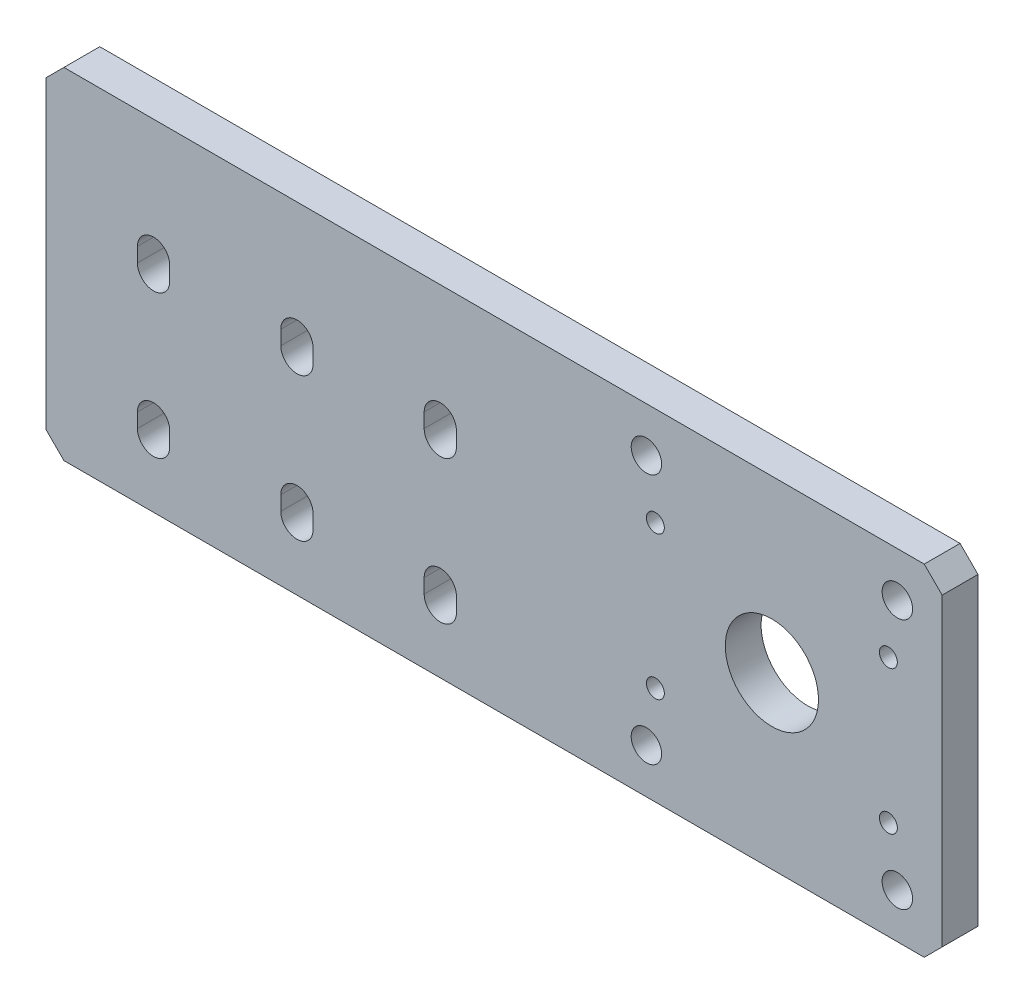
SolidWorks part; units mm, degrees
material "AISI 1045 钢，冷拔"
ref_plane "前视基准面" through (0, 0, 0) normal (0, 0, 1) x (1, 0, 0)
ref_plane "上视基准面" through (0, 0, 0) normal (0, 1, 0) x (1, 0, 0)
ref_plane "右视基准面" through (0, 0, 0) normal (1, 0, 0) x (0, 0, -1)
sketch "草图1" plane through (0, 0, 0) normal (0, 0, 1) x (1, 0, 0)
  line L1 (-125, 47.5) -> (125, 47.5)
  line L2 (-125, 47.5) -> (-125, -47.5)
  line L3 (-125, -47.5) -> (125, -47.5)
  line L4 (125, 47.5) -> (125, -47.5)
  line L5 (-125, 47.5) -> (125, -47.5) construction
  line L6 (-125, -47.5) -> (125, 47.5) construction
  point P0 (0, 0)
  dimension "D1" = 95
  dimension "D2" = 250
extrude "凸台-拉伸1" add sketch "草图1" along normal blind 10
sketch "草图3" plane through (0, 0, 10) normal (0, 0, 1) x (1, 0, 0)
  line L0 (-55, 17.5058) -> (-55, -69.5405) construction
  line L1 (125, -47.5) -> (125, 47.5) construction
  line L2 (-22.9727, -29.5) -> (-57.0867, -29.5) construction
  line L3 (-125, -47.5) -> (125, -47.5) construction
  line L4 (-55, -29.5) -> (-55, -25.5) construction
  line L5 (-59.5, -29.5) -> (-59.5, -25.5)
  line L6 (-50.5, -29.5) -> (-50.5, -25.5)
  arc A0 (-59.5, -29.5) -> (-50.5, -29.5) centre (-55, -29.5) ccw
  arc A1 (-50.5, -25.5) -> (-59.5, -25.5) centre (-55, -25.5) ccw
  point P10 (-55, -27.5)
  dimension "D4" = 4.5
  dimension "D1" = 180
  dimension "D2" = 18
  dimension "D3" = 4
extrude "切除-拉伸2" cut sketch "草图3" against normal through all
pattern_linear "阵列(线性)1" count 2 spacing 40 along (1, 0, 0) count 2 spacing 40 along (0, 1, 0) of "切除-拉伸2"
pattern_linear "阵列(线性)2" count 2 spacing 40 along (-1, 0, 0) count 2 spacing 40 along (0, 1, 0) of "切除-拉伸2"
chamfer "倒角1" distance 5 angle 45 4 edges at (125, -47.5, 5) (125, 47.5, 5) (-125, -47.5, 5) (-125, 47.5, 5)
sketch "草图10" plane through (0, 0, 10) normal (0, 0, 1) x (1, 0, 0)
  line L0 (5.5, 0) -> (-5.5, 0) construction
  line L1 (42.5, 35) -> (112.5, 35) construction
  line L2 (42.5, 35) -> (42.5, -35) construction
  line L3 (42.5, -35) -> (112.5, -35) construction
  line L4 (112.5, 35) -> (112.5, -35) construction
  line L5 (42.5, 35) -> (112.5, -35) construction
  line L6 (42.5, -35) -> (112.5, 35) construction
  line L7 (125, -42.5) -> (125, 42.5) construction
  point P0 (77.5, 0)
  dimension "D1" = 70
  dimension "D2" = 70
  dimension "D3" = 47.5
hole_wizard "M10 螺纹孔3" positions "3D草图3" profile "草图11" tap size "M10" standard "GB"
sketch3d "3D草图3"
  point P0 (42.5, 35, 10)
  point P3 (112.5, 35, 10)
  point P6 (112.5, -35, 10)
  point P9 (42.5, -35, 10)
sketch "草图11" plane through (42.5, 35, 10) normal (1, 0, 0) x (0, -1, 0)
  line L0 (0, 0) -> (0, 27.0537)
  line L1 (0, 27.0537) -> (4.25, 24.5)
  line L2 (4.25, 24.5) -> (4.25, 0)
  line L5 (4.25, 0) -> (0, 0)
  line L10 (0, 27.0537) -> (-4.25, 24.5) construction
  line L11 (0, -6.35) -> (0, 107.95) construction
  dimension "螺纹孔钻头直径" = 8.5
  dimension "螺纹孔钻头深度" = 24.5
  dimension "导头角度" = 118
cosmetic thread "孔螺蚊线9" parameters "D1"=10, "D2"=10
cosmetic thread "孔螺蚊线10" parameters "D1"=10, "D2"=10
cosmetic thread "孔螺蚊线11" parameters "D1"=10, "D2"=10
cosmetic thread "孔螺蚊线12" parameters "D1"=10, "D2"=10
sketch "草图12" plane through (0, 0, 10) normal (0, 0, 1) x (1, 0, 0)
  line L0 (42.5, 35) -> (112.5, -35) construction
  circle A0 centre (77.5, 0) radius 13
  dimension "D1" = 26
extrude "切除-拉伸5" cut sketch "草图12" against normal through all
sketch "草图13" plane through (0, 0, 0) normal (0, 0, -1) x (-1, 0, 0)
  line L0 (-45, -20) -> (-110, -20) construction
  line L1 (-110, -20) -> (-110, 20) construction
  line L2 (-110, 20) -> (-45, 20) construction
hole_wizard "M6 螺纹孔1" positions "3D草图4" profile "草图14" tap size "M6" standard "GB" end condition through all
sketch3d "3D草图4"
  point P0 (45, -20, 0)
  point P3 (110, -20, 0)
  point P6 (110, 20, 0)
  point P9 (45, 20, 0)
sketch "草图14" plane through (45, -20, 0) normal (1, 0, 0) x (0, 1, 0)
  line L0 (0, 0) -> (0, 10)
  line L1 (0, 10) -> (2.5, 10)
  line L2 (2.5, 10) -> (2.5, 0)
  line L5 (2.5, 0) -> (0, 0)
  line L11 (0, -6.35) -> (0, 107.95) construction
  dimension "通孔螺纹孔钻头直径" = 5
  dimension "通孔螺纹孔钻头深度" = 10
cosmetic thread "孔螺蚊线17" parameters "D2"=6
cosmetic thread "孔螺蚊线18" parameters "D2"=6
cosmetic thread "孔螺蚊线19" parameters "D2"=6
cosmetic thread "孔螺蚊线20" parameters "D2"=6
sketch "草图15" plane through (-125, 0, 0) normal (-1, 0, 0) x (0, 0, 1)
  line L0 (5, -37.5) -> (5, -17.5) construction
  line L1 (5, -17.5) -> (5, 2.5) construction
  line L2 (5, 2.5) -> (5, 22.5) construction
hole_wizard "M6 螺纹孔2" positions "3D草图5" profile "草图16" tap size "M6" standard "GB"
sketch3d "3D草图5"
  point P0 (-125, -37.5, 5)
  point P3 (-125, -17.5, 5)
  point P6 (-125, 2.5, 5)
  point P9 (-125, 22.5, 5)
sketch "草图16" plane through (-125, -37.5, 5) normal (0, 1, 0) x (0, 0, 1)
  line L0 (0, 0) -> (0, 16.5022)
  line L1 (0, 16.5022) -> (2.5, 15)
  line L2 (2.5, 15) -> (2.5, 0)
  line L5 (2.5, 0) -> (0, 0)
  line L10 (0, 16.5022) -> (-2.5, 15) construction
  line L11 (0, -6.35) -> (0, 107.95) construction
  dimension "螺纹孔钻头直径" = 5
  dimension "螺纹孔钻头深度" = 15
  dimension "导头角度" = 118
cosmetic thread "孔螺蚊线21" [suppressed] parameters "D1"=12, "D2"=6
cosmetic thread "孔螺蚊线22" [suppressed] parameters "D1"=12, "D2"=6
cosmetic thread "孔螺蚊线23" [suppressed] parameters "D1"=12, "D2"=6
cosmetic thread "孔螺蚊线24" [suppressed] parameters "D1"=12, "D2"=6
sketch "草图18" plane through (0, -47.5, 0) normal (0, -1, 0) x (1, 0, 0)
  line L0 (12, 5) -> (47, 5) construction
  line L1 (47, 5) -> (82, 5) construction
  line L2 (82, 5) -> (117, 5) construction
  point P4 (64.5, 5)
hole_wizard "M4 螺纹孔1" positions "3D草图6" profile "草图19" tap size "M4" standard "GB"
sketch3d "3D草图6"
  point P0 (117, -47.5, 5)
  point P9 (12, -47.5, 5)
  point P12 (64.5, -47.5, 5)
sketch "草图19" plane through (117, -47.5, 5) normal (1, 0, 0) x (0, 0, -1)
  line L0 (0, 0) -> (0, 11.0914)
  line L1 (0, 11.0914) -> (1.65, 10.1)
  line L2 (1.65, 10.1) -> (1.65, 0)
  line L5 (1.65, 0) -> (0, 0)
  line L10 (0, 11.0914) -> (-1.65, 10.1) construction
  line L11 (0, -6.35) -> (0, 107.95) construction
  dimension "螺纹孔钻头直径" = 3.3
  dimension "螺纹孔钻头深度" = 10.1
  dimension "导头角度" = 118
cosmetic thread "孔螺蚊线25" parameters "D1"=8, "D2"=4
cosmetic thread "孔螺蚊线26" parameters "D1"=8, "D2"=4
cosmetic thread "孔螺蚊线28" parameters "D1"=8, "D2"=4
